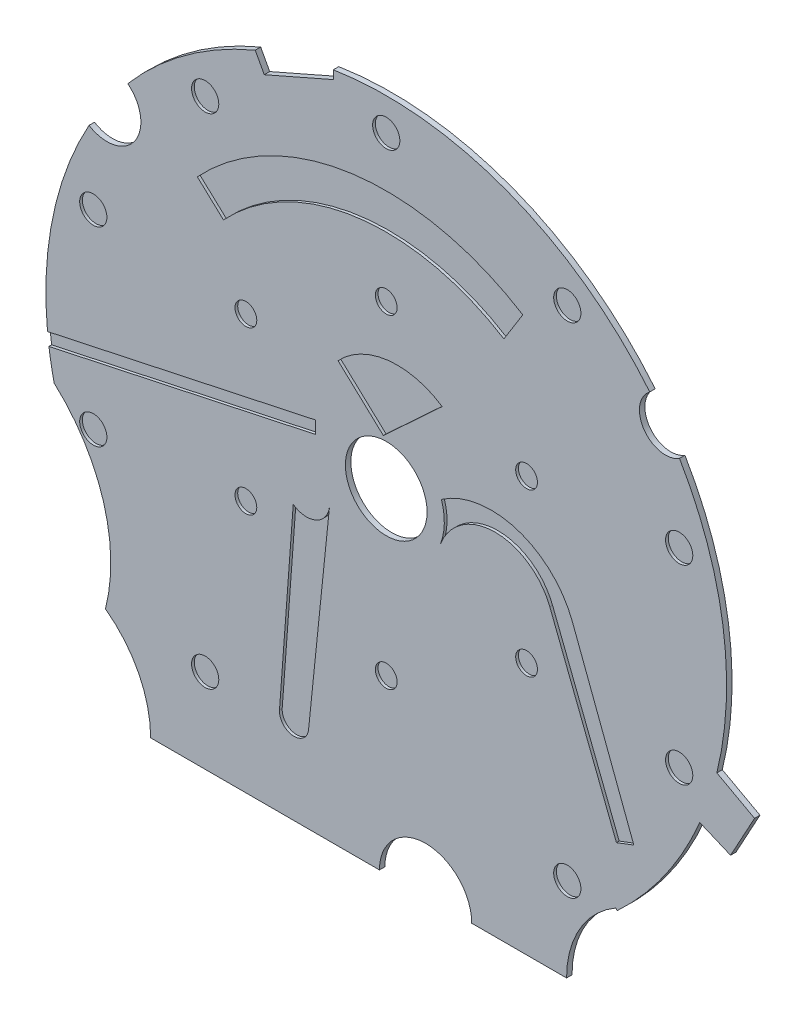
SolidWorks part; units mm, degrees
ref_plane "Front Plane" through (0, 0, 0) normal (0, 0, 1) x (1, 0, 0)
ref_plane "Top Plane" through (0, 0, 0) normal (0, 1, 0) x (1, 0, 0)
ref_plane "Right Plane" through (0, 0, 0) normal (1, 0, 0) x (0, 0, -1)
sketch "Sketch3" plane through (0, 0, 0) normal (0, 0, 1) x (1, 0, 0)
  line L0 (-8.6509, -12.2541) -> (-0.2487, -12.2541)
  line L1 (3.1404, -12.2541) -> (6.6229, -12.2541)
  line L2 (8.4263, -9.1259) -> (8.4798, -9.1838)
  line L3 (-4.8104, 11.5373) -> (-4.4792, 10.9227)
  line L4 (-4.4792, 10.9227) -> (-1.9433, 12.0354)
  line L5 (-1.9433, 12.0354) -> (-1.9433, 12.348)
  line L6 (12.1418, -2.9708) -> (13.5255, -3.7254)
  line L7 (13.5255, -3.7254) -> (12.645, -5.3401)
  line L8 (12.645, -5.3401) -> (11.5153, -4.863)
  arc A0 (8.4798, -9.1838) -> (11.5153, -4.863) centre (0, 0) ccw
  arc A1 (-0.2487, -12.2541) -> (3.1404, -12.2541) centre (1.4458, -12.2541) cw
  arc A2 (6.6229, -12.2541) -> (8.4263, -9.1259) centre (10.2377, -12.2541) cw
  arc A3 (-8.6509, -12.2541) -> (-10.3107, -8.9822) centre (-12.7055, -12.2541) ccw
  arc A4 (-4.8104, 11.5373) -> (-9.493, 8.1322) centre (0, 0) ccw
  arc A5 (-10.913, 6.0956) -> (-9.493, 8.1322) centre (-10.2537, 7.1492) ccw
  arc A6 (-10.913, 6.0956) -> (-12.1954, -2.7425) centre (0, 0) ccw
  arc A7 (9.6775, 7.9118) -> (10.77, 6.3449) centre (10.2537, 7.1492) ccw
  arc A8 (9.6775, 7.9118) -> (-1.9433, 12.348) centre (0, 0) ccw
  arc A9 (12.1418, -2.9708) -> (10.77, 6.3449) centre (0, 0) ccw
  arc A10 (-10.3107, -8.9822) -> (-12.1954, -2.7425) centre (-16.4274, -7.4253) ccw
  dimension "D1" = 25
extrude "Boss-Extrude2" add sketch "Sketch3" along normal blind 0.2
sketch "Sketch4" plane through (0, 0, 0.2) normal (0, 0, 1) x (1, 0, 0)
  circle A0 centre (0, 0) radius 1.5
  dimension "D1" = 3
extrude "Cut-Extrude1" cut sketch "Sketch4" against normal blind 0.2
sketch "Sketch5" plane through (0, 0, 0.2) normal (0, 0, 1) x (1, 0, 0)
  circle A0 centre (0, 11.3119) radius 0.5
  circle A1 centre (6.6489, 9.1515) radius 0.5
  circle A2 centre (10.7582, 3.4956) radius 0.5
  circle A3 centre (10.7582, -3.4956) radius 0.5
  circle A4 centre (6.6489, -9.1515) radius 0.5
  circle A6 centre (-6.6489, -9.1515) radius 0.5
  circle A7 centre (-10.7582, -3.4956) radius 0.5
  circle A8 centre (-10.7582, 3.4956) radius 0.5
  circle A9 centre (-6.6489, 9.1515) radius 0.5
  circle A10 centre (0, -11.3119) radius 0.5 [skipped]
  point P22 (0, 0)
  dimension "D1" = 1
  dimension "D2" = 10
extrude "Cut-Extrude2" cut sketch "Sketch5" against normal blind 0.1
sketch "Sketch6" plane through (0, 0, 0.2) normal (0, 0, 1) x (1, 0, 0)
  circle A0 centre (0, 5.9513) radius 0.4
  circle A1 centre (5.154, 2.9757) radius 0.4
  circle A2 centre (5.154, -2.9757) radius 0.4
  circle A3 centre (0, -5.9513) radius 0.4
  circle A4 centre (-5.154, -2.9757) radius 0.4
  circle A5 centre (-5.154, 2.9757) radius 0.4
  point P15 (0, 0)
  dimension "D1" = 0.8
  dimension "D2" = 6
extrude "Cut-Extrude3" cut sketch "Sketch6" against normal blind 0.1
sketch "Sketch7" plane through (0, 0, 0.2) normal (0, 0, 1) x (1, 0, 0)
  line L0 (-0.1057, 1.6339) -> (-1.7705, 3.1815)
  line L1 (2.0548, 3.6361) -> (-0.1057, 1.6339)
  line L2 (-2.5966, 0.8828) -> (-13.2134, -1.3907)
  line L3 (-13.2134, -1.3907) -> (-13.2134, -1.8496)
  line L4 (-13.2134, -1.8496) -> (-2.5966, 0.4239)
  line L5 (-2.5966, 0.4239) -> (-2.5966, 0.8828)
  line L6 (-5.9772, 5.5546) -> (-6.9374, 6.4469)
  line L7 (4.3215, 6.9213) -> (5.0157, 8.0332)
  line L8 (-3.415, -2.21) -> (-3.92, -8.9972)
  line L9 (-2.8508, -9.0767) -> (-2.0818, -1.604)
  line L10 (6.8369, -0.8171) -> (9.0925, -6.7926)
  line L11 (9.0925, -6.7926) -> (8.4541, -7.0336)
  line L12 (8.4541, -7.0336) -> (6.008, -0.7576)
  arc A1 (-1.7705, 3.1815) -> (2.0548, 3.6361) centre (0.41, 1.1545) cw
  arc A2 (5.0157, 8.0332) -> (-6.9374, 6.4469) centre (0, 0) ccw
  arc A3 (4.7132, 7.5487) -> (-6.519, 6.0581) centre (0, 0) ccw
  arc A4 (4.3215, 6.9213) -> (-5.9772, 5.5546) centre (0, 0) ccw
  arc A5 (-3.92, -8.9972) -> (-2.8508, -9.0767) centre (-3.3854, -9.037) ccw
  arc A6 (-2.0818, -1.604) -> (-3.415, -2.21) centre (-2.9256, -1.5172) cw
  arc A7 (2.0257, 0.6683) -> (6.8369, -0.8171) centre (3.8544, -1.9429) cw
  arc A8 (1.9908, -0.7662) -> (6.008, -0.7576) centre (4.001, -1.5398) cw
  arc A9 (1.9908, -0.7662) -> (2.0257, 0.6683) centre (0, 0) ccw
extrude "Cut-Extrude6" cut sketch "Sketch7" against normal blind 0.1 contours A3 L7 A2 L6 | A4 L7 A3 L6 | L4 L5 L2 L3 | L9 A6 L8 A5 | A1 L0 L1 | A9 A8 L12 L11 L10 A7
